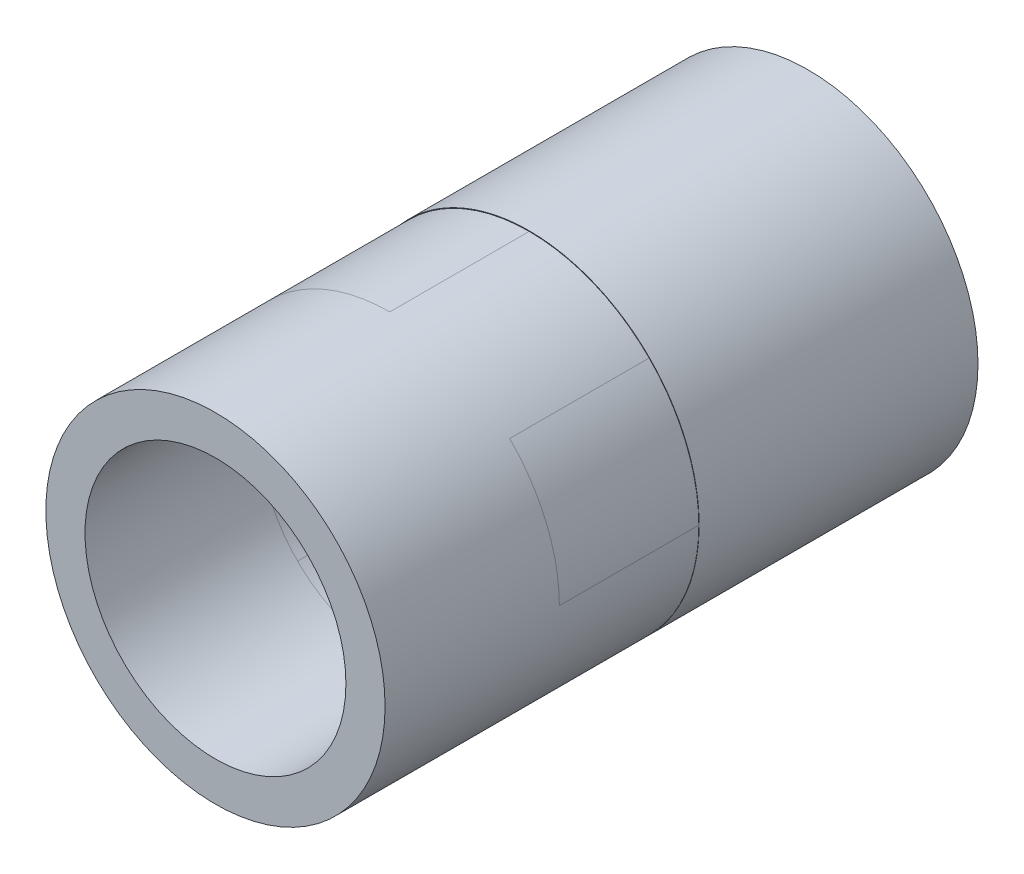
from build123d import *
from build123d.topology import SkipClean

# Parameters (mm, degrees)
BOSS_EXTRUDE1_DEPTH      = 4
BOSS_EXTRUDE1_DEPTH_BACK = 4
SKETCH1_R                = 4.872852562
SKETCH1_R_2              = 3.75
BOSS_EXTRUDE2_DEPTH      = 4
SKETCH4_R                = 4.865070387
SKETCH4_R_2              = 3.742217825
BOSS_EXTRUDE3_DEPTH      = 5
BOSS_EXTRUDE4_START      = 4
BOSS_EXTRUDE4_DEPTH      = 4


with BuildPart() as part:
    # Sketch1 → Boss-Extrude1 (new, two sides: drawn at the far end of the back side and taken through both)
    with BuildSketch(Plane.XY.offset(-BOSS_EXTRUDE1_DEPTH_BACK)):
        with Locations((1.501e-06, 0.007782175)):
            Circle(SKETCH1_R)
        with Locations((1.501e-06, 0.007782175)):
            Circle(SKETCH1_R_2, mode=Mode.SUBTRACT)
    extrude(amount=BOSS_EXTRUDE1_DEPTH + BOSS_EXTRUDE1_DEPTH_BACK)

    # Sketch3 → Boss-Extrude2 (add)
    with BuildSketch(Plane.XY.offset(4)):
        with BuildLine():
            Line((0, 3.757782175), (0, 4.865070387))
            ThreePointArc((0, 4.865070387), (-1.861781834, 4.494738955), (-3.440124262, 3.440124262))
            Line((-3.440124262, 3.440124262), (-2.65553791, 2.65553791))
            ThreePointArc((-2.65553791, 2.65553791), (-1.437604143, 3.471276077), (0, 3.757782175))
        make_face()
        with BuildLine():
            Line((3.757782175, 0), (4.865070387, 0))
            ThreePointArc((4.865070387, 0), (4.494738955, 1.861781834), (3.440124262, 3.440124262))
            Line((3.440124262, 3.440124262), (2.65553791, 2.65553791))
            ThreePointArc((2.65553791, 2.65553791), (3.471276077, 1.437604143), (3.757782175, 0))
        make_face()
        with BuildLine():
            Line((0, -3.757782175), (0, -4.865070387))
            ThreePointArc((0, -4.865070387), (1.861781834, -4.494738955), (3.440124262, -3.440124262))
            Line((3.440124262, -3.440124262), (2.65553791, -2.65553791))
            ThreePointArc((2.65553791, -2.65553791), (1.437604143, -3.471276077), (0, -3.757782175))
        make_face()
        with BuildLine():
            Line((-3.757782175, 0), (-4.865070387, 0))
            ThreePointArc((-4.865070387, 0), (-4.494738955, -1.861781834), (-3.440124262, -3.440124262))
            Line((-3.440124262, -3.440124262), (-2.65553791, -2.65553791))
            ThreePointArc((-2.65553791, -2.65553791), (-3.471276077, -1.437604143), (-3.757782175, 0))
        make_face()
    extrude(amount=BOSS_EXTRUDE2_DEPTH)


with BuildPart() as body_2:
    # Sketch4 → Boss-Extrude3 (new body)
    with BuildSketch(Plane.XY.offset(8)):
        Circle(SKETCH4_R)
        Circle(SKETCH4_R_2, mode=Mode.SUBTRACT)
    extrude(amount=BOSS_EXTRUDE3_DEPTH)

    # Sketch5 → Boss-Extrude4 (add)
    with SkipClean():  # the faces are left unmerged after this step: merging them gives an invalid solid
        with BuildSketch(Plane(origin=(0, 0, 8), x_dir=(-1, 0, 0), z_dir=(0, 0, -1)).offset(BOSS_EXTRUDE4_START)):
            with BuildLine():
                Line((0, 3.757782175), (0, 4.865070387))
                ThreePointArc((0, 4.865070387), (-1.861781834, 4.494738955), (-3.440124261, 3.440124261))
                Line((-3.440124262, 3.440124262), (-2.657153258, 2.657153258))
                ThreePointArc((-2.657153258, 2.657153258), (-1.438040981, 3.471738039), (0, 3.757782175))
            make_face()
            with BuildLine():
                ThreePointArc((2.657153258, 2.657153258), (3.471738039, 1.438040981), (3.757782175, 0))
                Line((3.757782175, 0), (4.865070387, 0))
                ThreePointArc((4.865070387, 0), (4.494738955, 1.861781834), (3.440124262, 3.440124262))
                Line((3.440124262, 3.440124262), (2.657153258, 2.657153258))
            make_face()
            with BuildLine():
                ThreePointArc((-4.865070387, 0), (-4.494738955, -1.861781834), (-3.440124261, -3.440124261))
                Line((-3.440124262, -3.440124262), (-2.657153258, -2.657153258))
                ThreePointArc((-2.657153258, -2.657153258), (-3.471738039, -1.438040981), (-3.757782175, 0))
                Line((-3.757782175, 0), (-4.865070387, 0))
            make_face()
            with BuildLine():
                ThreePointArc((0, -4.865070387), (1.861781834, -4.494738955), (3.440124262, -3.440124262))
                Line((3.440124262, -3.440124262), (2.657153258, -2.657153258))
                ThreePointArc((2.657153258, -2.657153258), (1.438040981, -3.471738039), (0, -3.757782175))
                Line((0, -3.757782175), (0, -4.865070387))
            make_face()
        extrude(amount=-BOSS_EXTRUDE4_DEPTH)


solid = Compound([part.part, body_2.part])
